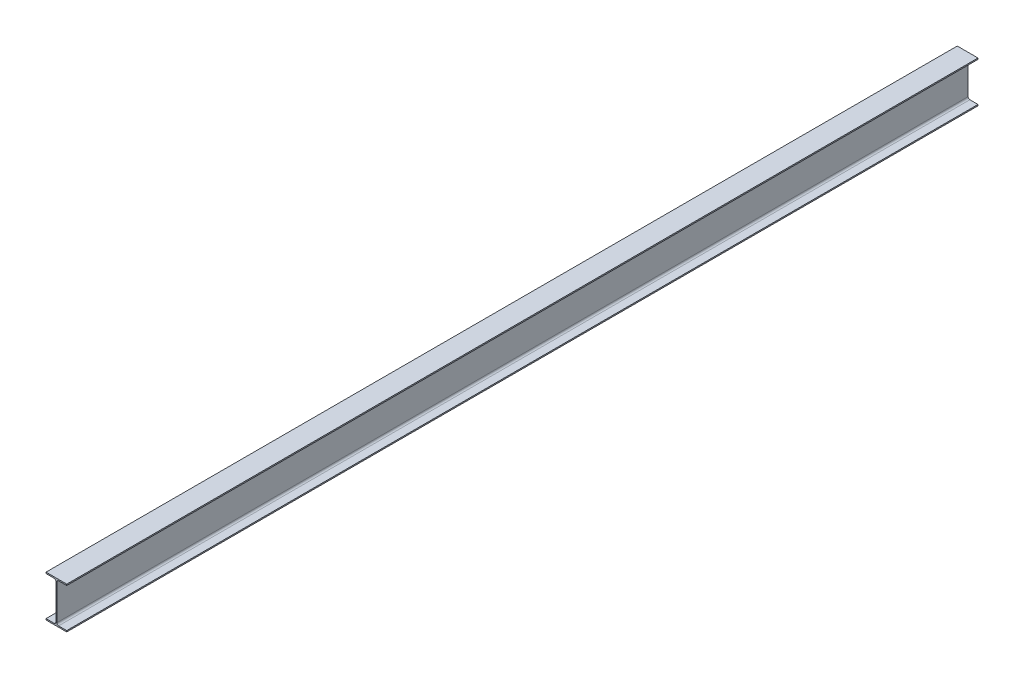
SolidWorks part; units mm, degrees
ref_plane "Front Plane" through (0, 0, 0) normal (0, 0, 1) x (1, 0, 0)
ref_plane "Top Plane" through (0, 0, 0) normal (0, 1, 0) x (1, 0, 0)
ref_plane "Right Plane" through (0, 0, 0) normal (1, 0, 0) x (0, 0, -1)
other "Configuration Table"
sketch "Sketch1" plane through (0, 0, 0) normal (0, 0, 1) x (1, 0, 0)
  line L0 (0, 0) -> (0, 300) construction
  line L1 (75, 0) -> (-75, 0)
  line L2 (-75, 0) -> (-75, 9)
  line L3 (-75, 9) -> (-16.25, 9)
  line L4 (3.25, 22) -> (3.25, 278)
  line L6 (-75, 291) -> (-75, 300)
  line L7 (-75, 300) -> (75, 300)
  line L8 (-3.25, 22) -> (-3.25, 278)
  line L9 (75, 291) -> (75, 300)
  line L10 (16.25, 291) -> (75, 291)
  line L11 (75, 9) -> (16.25, 9)
  line L12 (75, 0) -> (75, 9)
  line L13 (-16.25, 291) -> (-75, 291)
  arc A0 (16.25, 9) -> (3.25, 22) centre (16.25, 22) cw
  arc A1 (-3.25, 22) -> (-16.25, 9) centre (-16.25, 22) cw
  arc A2 (3.25, 278) -> (16.25, 291) centre (16.25, 278) cw
  arc A3 (-3.25, 278) -> (-16.25, 291) centre (-16.25, 278) ccw
  point P18 (3.25, 9)
  point P21 (-3.25, 9)
  point P24 (3.25, 291)
  point P27 (-3.25, 291)
  dimension "D6" = 13
  dimension "D1" = 300
  dimension "D2" = 150
  dimension "D3" = 6.5
  dimension "D4" = 9
  dimension "D5" = 9
extrude "Boss-Extrude1" add sketch "Sketch1" along normal blind 6592
